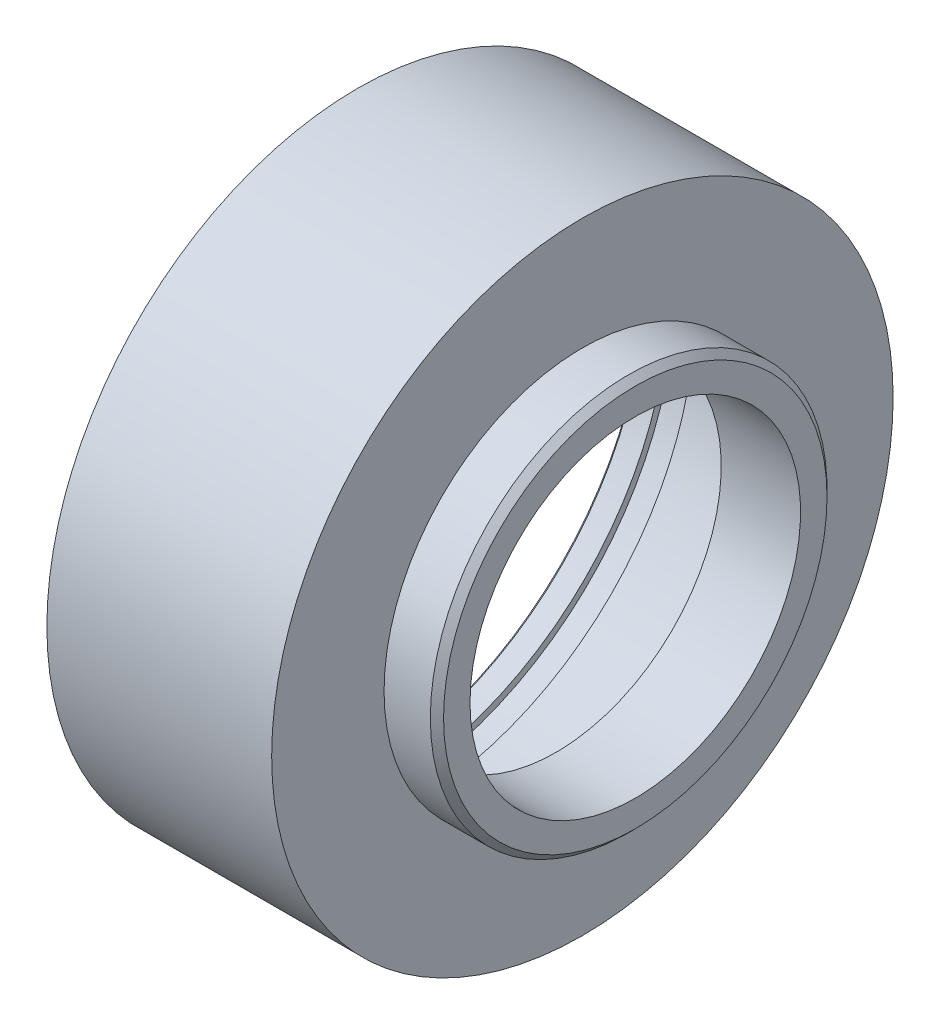
from build123d import *

# Parameters (mm, degrees)
CHAMFER_1_SIZE = 0.25
CHAMFER_2_SIZE = 0.5


with BuildPart() as part:
    # 草图1 → 旋转1 (revolve)
    with BuildSketch(Plane.XY, mode=Mode.PRIVATE) as revolve_1_sk:
        Polygon((2.179589421, 21.5), (4.179589421, 21.5), (4.179589421, 22), (6.179589421, 22), (6.179589421, 21.5), (13.179589421, 21.5), (13.179589421, 21), (17.179589421, 21), (17.179589421, 12.5), (23.179589421, 12.5), (23.179589421, 15), (19.179589421, 15), (19.179589421, 23.5), (2.179589421, 23.5), align=None)
    revolve(revolve_1_sk.sketch.rotate(Axis((0, 0, 0), (1, 0, 0)), 90), axis=Axis((0, 0, 0), (1, 0, 0)))

    # 倒角1
    chamfer_1_edges = [part.edges().sort_by_distance(p)[0] for p in [
        (2.179589421, 0, -21.5),
    ]]
    chamfer(chamfer_1_edges, length=CHAMFER_1_SIZE)

    # 倒角2
    chamfer_2_edges = [part.edges().sort_by_distance(p)[0] for p in [
        (23.179589421, 0, -15),
    ]]
    chamfer(chamfer_2_edges, length=CHAMFER_2_SIZE)


solid = part.part
